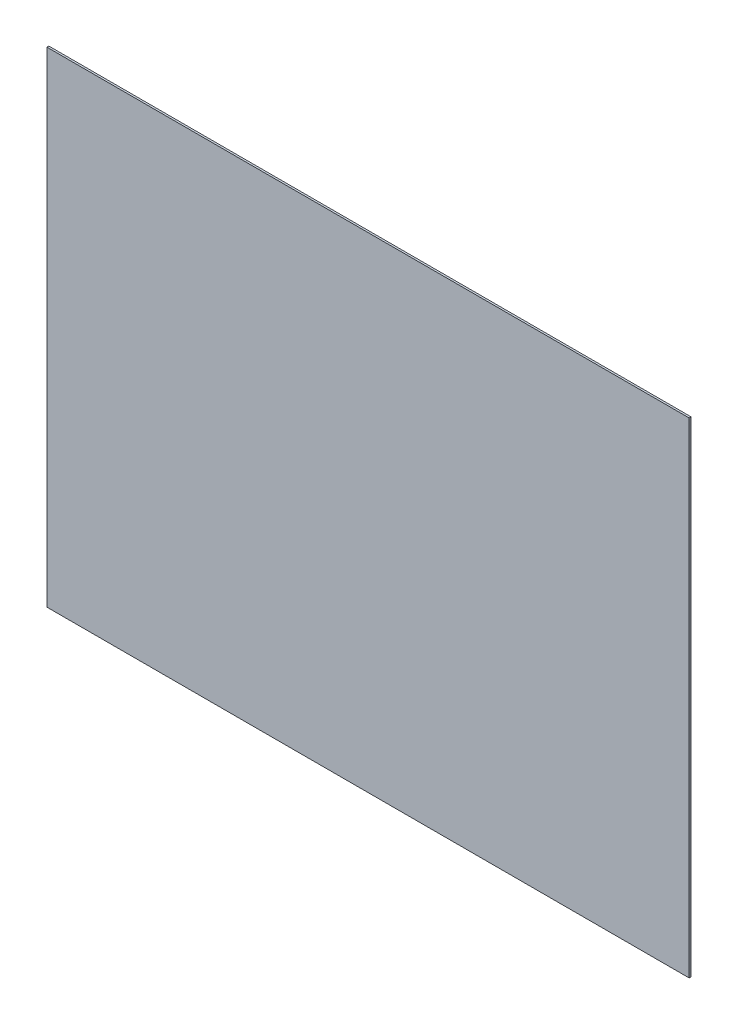
SolidWorks part; units mm, degrees
ref_plane "Front Plane" through (0, 0, 0) normal (0, 0, 1) x (1, 0, 0)
ref_plane "Top Plane" through (0, 0, 0) normal (0, 1, 0) x (1, 0, 0)
ref_plane "Right Plane" through (0, 0, 0) normal (1, 0, 0) x (0, 0, -1)
sketch "Sketch1" plane through (0, 0, 0) normal (0, 0, 1) x (1, 0, 0)
  line L1 (0, 0) -> (1000, 0)
  line L2 (0, 0) -> (0, 755)
  line L3 (0, 755) -> (1000, 755)
  line L4 (1000, 0) -> (1000, 755)
  dimension "D1" = 1000
  dimension "D2" = 755
extrude "Boss-Extrude1" add sketch "Sketch1" along normal blind 3
